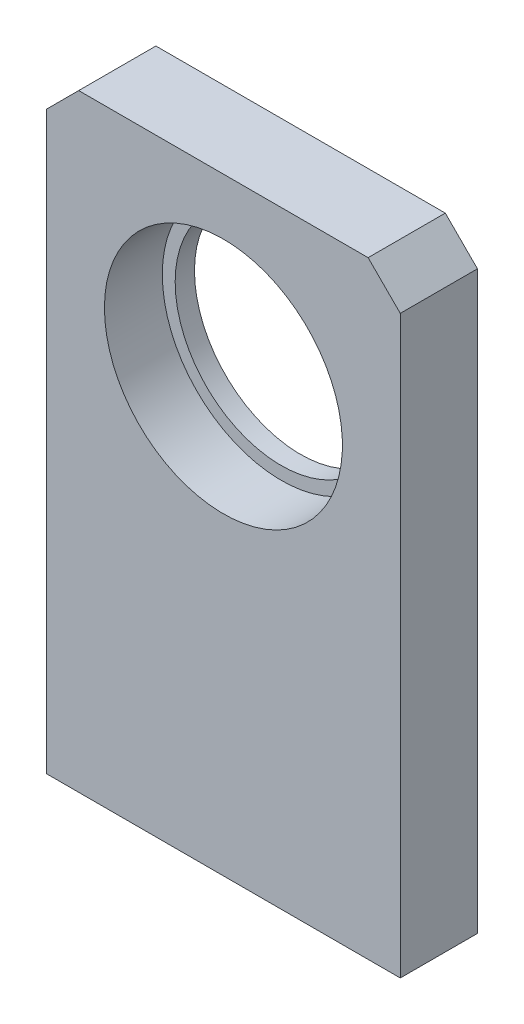
SolidWorks part; units mm, degrees
ref_plane "前视基准面" through (0, 0, 0) normal (0, 0, 1) x (1, 0, 0)
ref_plane "上视基准面" through (0, 0, 0) normal (0, 1, 0) x (1, 0, 0)
ref_plane "右视基准面" through (0, 0, 0) normal (1, 0, 0) x (0, 0, -1)
sketch "草图1" plane through (0, 0, 0) normal (0, 0, 1) x (1, 0, 0)
  line L1 (-27.5, -47.25) -> (27.5, -47.25)
  line L2 (-27.5, -47.25) -> (-27.5, 47.25)
  line L3 (-27.5, 47.25) -> (27.5, 47.25)
  line L4 (27.5, -47.25) -> (27.5, 47.25)
  line L5 (-27.5, -47.25) -> (27.5, 47.25) construction
  line L6 (-27.5, 47.25) -> (27.5, -47.25) construction
  point P0 (0, 0)
  dimension "D1" = 94.5
  dimension "D2" = 55
extrude "凸台-拉伸1" add sketch "草图1" along normal blind 12
sketch "草图3" plane through (0, 0, 0) normal (0, 0, -1) x (-1, 0, 0)
  line L0 (-27.5, 47.25) -> (27.5, 47.25) construction
  line L1 (27.5, -47.25) -> (17.5, -47.25)
  line L2 (27.5, -47.25) -> (27.5, 47.25)
  line L3 (27.5, 47.25) -> (17.5, 47.25)
  line L4 (17.5, -47.25) -> (17.5, 47.25)
  line L6 (-27.5, -47.25) -> (-17.5, -47.25)
  line L7 (-27.5, -47.25) -> (-27.5, 47.25)
  line L8 (-27.5, 47.25) -> (-17.5, 47.25)
  line L9 (-17.5, -47.25) -> (-17.5, 47.25)
  dimension "D1" = 10
extrude "切除-拉伸2" [suppressed] cut sketch "草图3" against normal blind 1.5
sketch "草图4" plane through (0, 47.25, 0) normal (0, 1, 0) x (1, 0, 0)
  line L0 (27.5, -12) -> (-27.5, -12) construction
  line L1 (-15, 0) -> (15, 0)
  line L2 (-15, 0) -> (-15, -12)
  line L3 (-15, -12) -> (15, -12)
  line L4 (15, 0) -> (15, -12)
  line L5 (-15, 0) -> (15, -12) construction
  line L6 (-15, -12) -> (15, 0) construction
  line L7 (27.5, 0) -> (-27.5, 0) construction
  point P0 (0, -6)
  dimension "D1" = 30
extrude "切除-拉伸3" [suppressed] cut sketch "草图4" against normal blind 8
sketch "草图5" plane through (0, 0, 0) normal (0, 0, -1) x (-1, 0, 0)
  circle A0 centre (0, 20) radius 18.5
  dimension "D1" = 37
  dimension "D2" = 20
extrude "切除-拉伸4" cut sketch "草图5" against normal up to next
chamfer "倒角1" distance 5 angle 45 2 edges at (-27.5, 47.25, 6) (27.5, 47.25, 6)
sketch "草图6" plane through (0, 0, 0) normal (0, 0, -1) x (-1, 0, 0)
  circle A0 centre (0, 20) radius 16.5
  circle A1 centre (0, 20) radius 18.5 construction
  circle A2 centre (0, 20) radius 18.5
  dimension "D1" = 33
extrude "凸台-拉伸2" add sketch "草图6" against normal blind 3
